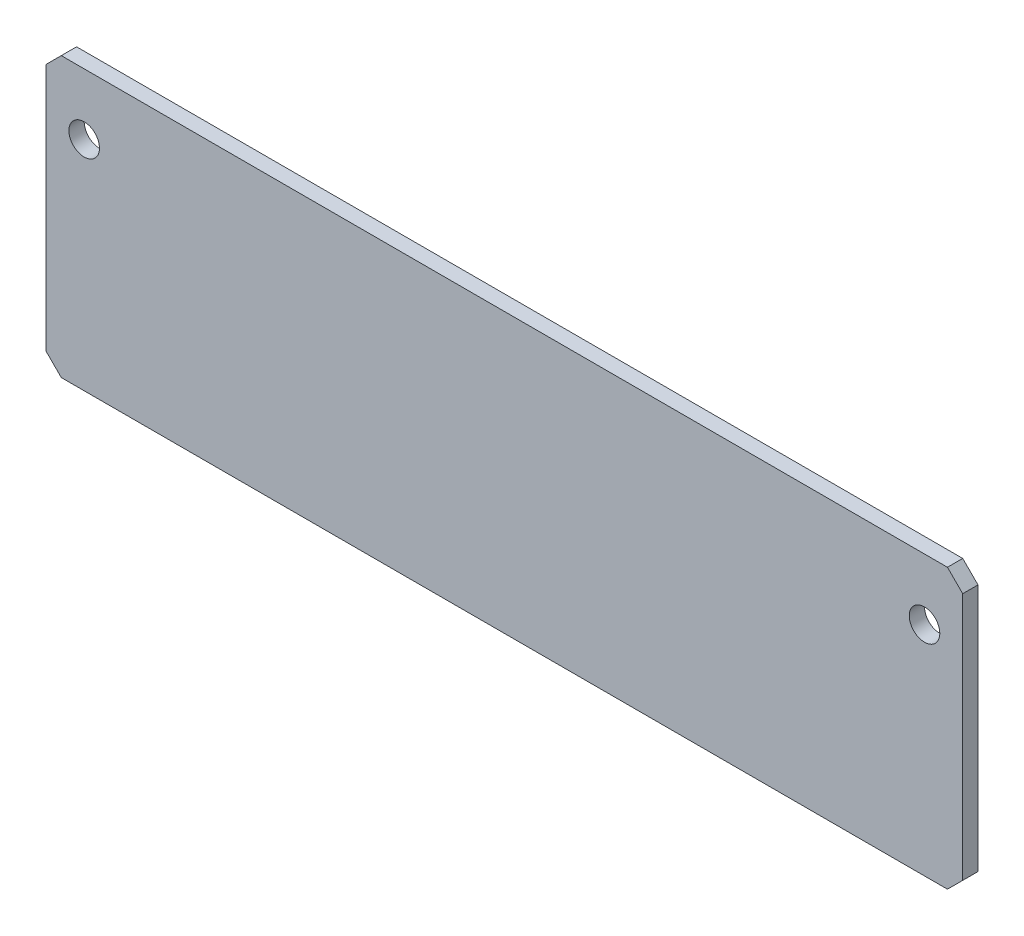
from build123d import *

# Parameters (mm, degrees)
SKETCH1_W               = 1200
SKETCH1_H               = 365
BOSS_EXTRUDE1_DEPTH     = 20
CUT_EXTRUDE1_DEPTH      = 628.460158098
CUT_EXTRUDE1_DEPTH_BACK = 628.460158098
SKETCH2_R               = 20
CHAMFER1_SIZE           = 20
CHAMFER2_SIZE           = 20


with BuildPart() as part:
    # Sketch1 → Boss-Extrude1 (new body)
    with BuildSketch(Plane.XY):
        Rectangle(SKETCH1_W, SKETCH1_H)
    extrude(amount=BOSS_EXTRUDE1_DEPTH)

    # Sketch2 → Cut-Extrude1 (cut, two sides: drawn at the far end of the back side and taken through both)
    with BuildSketch(Plane.XY.offset(20).offset(-CUT_EXTRUDE1_DEPTH_BACK)):
        with Locations((-550, 102.5)):
            Circle(SKETCH2_R)
        with Locations((550, 102.5)):
            Circle(SKETCH2_R)
    extrude(amount=CUT_EXTRUDE1_DEPTH + CUT_EXTRUDE1_DEPTH_BACK, mode=Mode.SUBTRACT)

    # Chamfer1
    chamfer1_edges = [part.edges().sort_by_distance(p)[0] for p in [
        (-600, 182.5, 10),
        (600, 182.5, 10),
    ]]
    chamfer(chamfer1_edges, length=CHAMFER1_SIZE)

    # Chamfer2
    chamfer2_edges = [part.edges().sort_by_distance(p)[0] for p in [
        (600, -182.5, 10),
        (-600, -182.5, 10),
    ]]
    chamfer(chamfer2_edges, length=CHAMFER2_SIZE)


solid = part.part
